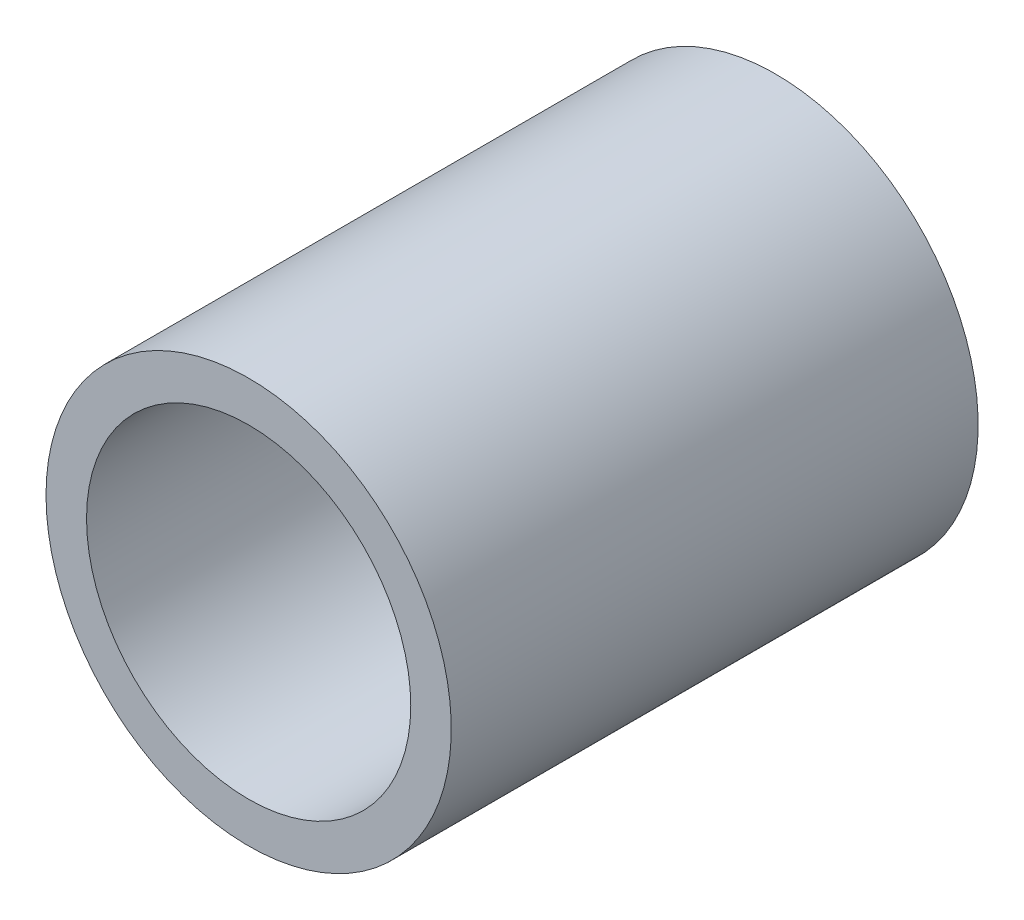
from build123d import *

# Parameters (mm, degrees)
SKETCH1_R           = 10
SKETCH1_R_2         = 8
BOSS_EXTRUDE1_DEPTH = 13


with BuildPart() as part:
    # Sketch1 → Boss-Extrude1 (new, symmetric)
    with BuildSketch(Plane.XY):
        with Locations(Location((0, 0, 0), (0, 0, 180))):
            Circle(SKETCH1_R)
        with Locations(Location((0, 0, 0), (0, 0, 180))):
            Circle(SKETCH1_R_2, mode=Mode.SUBTRACT)
    extrude(amount=BOSS_EXTRUDE1_DEPTH, both=True)


solid = part.part
